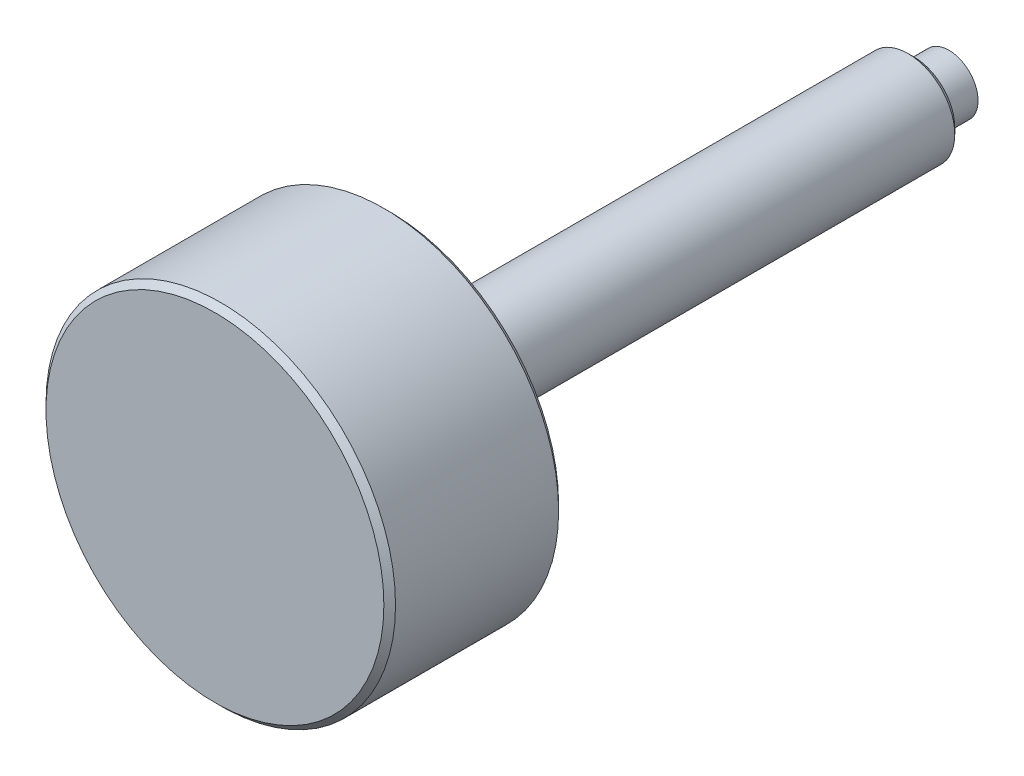
SolidWorks part; units mm, degrees
material "S45C"
ref_plane "Front Plane" through (0, 0, 0) normal (0, 0, 1) x (1, 0, 0)
ref_plane "Top Plane" through (0, 0, 0) normal (0, 1, 0) x (1, 0, 0)
ref_plane "Right Plane" through (0, 0, 0) normal (1, 0, 0) x (0, 0, -1)
sketch "Sketch1" plane through (0, 0, 0) normal (0, 0, 1) x (1, 0, 0)
  circle A0 centre (0, 0) radius 4
  dimension "D1" = 8
extrude "Boss-Extrude1" add sketch "Sketch1" along normal blind 45
cosmetic thread "Cosmetic Thread1" parameters "D2"=6.891
sketch "Sketch2" plane through (0, 0, 45) normal (0, 0, 1) x (1, 0, 0)
  circle A0 centre (0, 0) radius 15
  dimension "D1" = 30
extrude "Boss-Extrude2" add sketch "Sketch2" along normal blind 15
sketch "Sketch3" plane through (0, 0, 0) normal (0, 0, -1) x (-1, 0, 0)
  circle A0 centre (0, 0) radius 2.5
  dimension "D1" = 5
extrude "Cut-Extrude1" cut sketch "Sketch3" against normal blind 4
sketch "Sketch4" plane through (0, 0, 4) normal (0, 0, -1) x (-1, 0, 0)
  circle A0 centre (0, 0) radius 2.5
extrude "Boss-Extrude3" add sketch "Sketch4" along normal blind 7 separate body
chamfer "Chamfer1" distance 0.5 angle 45 3 edges at (4, 0, 0) (15, 0, 45) (15, 0, 60)
